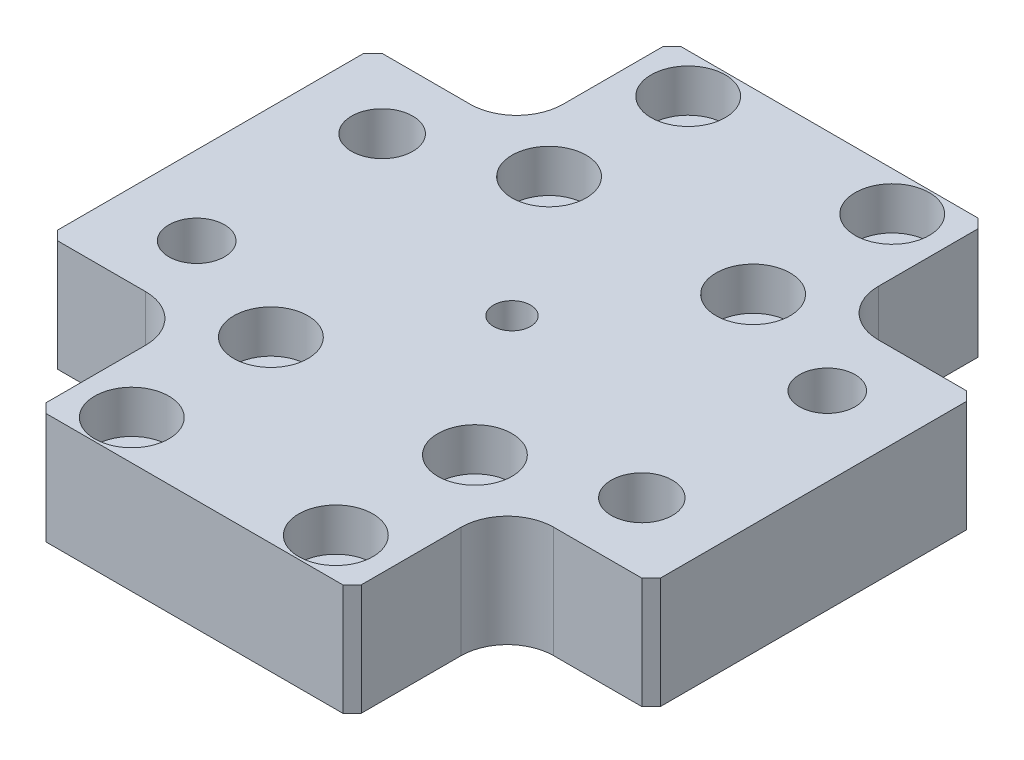
from build123d import *

# Parameters (mm, degrees)
SKETCH_1_W                   = 65
SKETCH_1_H                   = 68.5
SKETCH_1_R                   = 2
EXTRUDE_1_DEPTH              = 6
HOLE_WIZARD_M6_1_D           = 6.6
HOLE_WIZARD_M6_1_CBORE_D     = 11
HOLE_WIZARD_M6_1_CBORE_DEPTH = 6.8
HOLE_WIZARD_M4_1_D           = 4.5
HOLE_WIZARD_M4_1_CBORE_D     = 8
HOLE_WIZARD_M4_1_CBORE_DEPTH = 4.6
CUT_EXTRUDE_1_DEPTH          = 49.716655263
CUT_EXTRUDE_1_DEPTH_BACK     = 49.716655263
F_6_0MM_1_D                  = 6
CHAMFER_1_SIZE               = 1
SKETCH_9_R                   = 7.5
CUT_EXTRUDE_2_DEPTH          = 2


with BuildPart() as part:
    # 草图1 → 凸台-拉伸1 (new, symmetric)
    with BuildSketch(Plane(origin=(0, 0, 0), x_dir=(1, 0, 0), z_dir=(0, 1, 0))):
        Rectangle(SKETCH_1_W, SKETCH_1_H)
        with Locations(Location((0, 0, 0), (0, 0, 270))):
            Circle(SKETCH_1_R, mode=Mode.SUBTRACT)
    extrude(amount=EXTRUDE_1_DEPTH, both=True)

    # M6 六角圆柱头螺钉的柱形沉头孔1 (through all)
    with Locations(Plane.XZ.offset(6)):
        with Locations((-24, -10), (24, 10)):
            CounterBoreHole(HOLE_WIZARD_M6_1_D / 2, HOLE_WIZARD_M6_1_CBORE_D / 2, HOLE_WIZARD_M6_1_CBORE_DEPTH)

    # M4 六角圆柱头螺钉的柱形沉头孔1 (through all)
    with Locations(Plane(origin=(0, 6, 0), x_dir=(1, 0, 0), z_dir=(0, 1, 0))):
        with Locations((-11, -15), (-11, -30), (11, -30), (11, -15), (11, 15), (11, 30), (-11, 30), (-11, 15)):
            CounterBoreHole(HOLE_WIZARD_M4_1_D / 2, HOLE_WIZARD_M4_1_CBORE_D / 2, HOLE_WIZARD_M4_1_CBORE_DEPTH)

    # 草图6 → 切除-拉伸1 (cut, two sides: drawn at the far end of the back side and taken through both)
    with BuildSketch(Plane(origin=(0, 6, 0), x_dir=(1, 0, 0), z_dir=(0, 1, 0)).offset(-CUT_EXTRUDE_1_DEPTH_BACK)):
        with BuildLine():
            Line((-32.5, 34.25), (-17, 34.25))
            Line((-17, 34.25), (-17, 22.5))
            ThreePointArc((-17, 22.5), (-18.464466094, 18.964466094), (-22, 17.5))
            Line((-22, 17.5), (-32.5, 17.5))
            Line((-32.5, 17.5), (-32.5, 34.25))
        make_face()
        with BuildLine():
            Line((-17, -34.25), (-17, -22.5))
            ThreePointArc((-17, -22.5), (-18.464466094, -18.964466094), (-22, -17.5))
            Line((-22, -17.5), (-32.5, -17.5))
            Line((-32.5, -17.5), (-32.5, -34.25))
            Line((-32.5, -34.25), (-17, -34.25))
        make_face()
        with BuildLine():
            Line((32.5, -34.25), (17, -34.25))
            Line((17, -34.25), (17, -22.5))
            ThreePointArc((17, -22.5), (18.464466094, -18.964466094), (22, -17.5))
            Line((22, -17.5), (32.5, -17.5))
            Line((32.5, -17.5), (32.5, -34.25))
        make_face()
        with BuildLine():
            Line((17, 34.25), (17, 22.5))
            ThreePointArc((17, 22.5), (18.464466094, 18.964466094), (22, 17.5))
            Line((22, 17.5), (32.5, 17.5))
            Line((32.5, 17.5), (32.5, 34.25))
            Line((32.5, 34.25), (17, 34.25))
        make_face()
    extrude(amount=CUT_EXTRUDE_1_DEPTH + CUT_EXTRUDE_1_DEPTH_BACK, mode=Mode.SUBTRACT)

    # Ø6.0mm 暗销孔1 (through all)
    with Locations(Plane(origin=(0, -6, 0), x_dir=(-1, 0, 0), z_dir=(0, -1, 0))):
        with Locations((-24, 10), (24, -10)):
            Hole(F_6_0MM_1_D / 2)

    # 倒角1
    chamfer_1_edges = [part.edges().sort_by_distance(p)[0] for p in [
        (0, -6, -2),
        (17, 0, -34.25),
        (32.5, 0, -17.5),
        (32.5, 0, 17.5),
        (17, 0, 34.25),
        (-17, 0, 34.25),
        (-32.5, 0, 17.5),
        (-32.5, 0, -17.5),
        (-17, 0, -34.25),
    ]]
    chamfer(chamfer_1_edges, length=CHAMFER_1_SIZE)

    # 草图9 → 切除-拉伸2 (cut)
    with BuildSketch(Plane.XZ.offset(6)):
        with Locations(Location((0, 0, 0), (0, 0, 270))):
            Circle(SKETCH_9_R)
    extrude(amount=-CUT_EXTRUDE_2_DEPTH, mode=Mode.SUBTRACT)


solid = part.part
